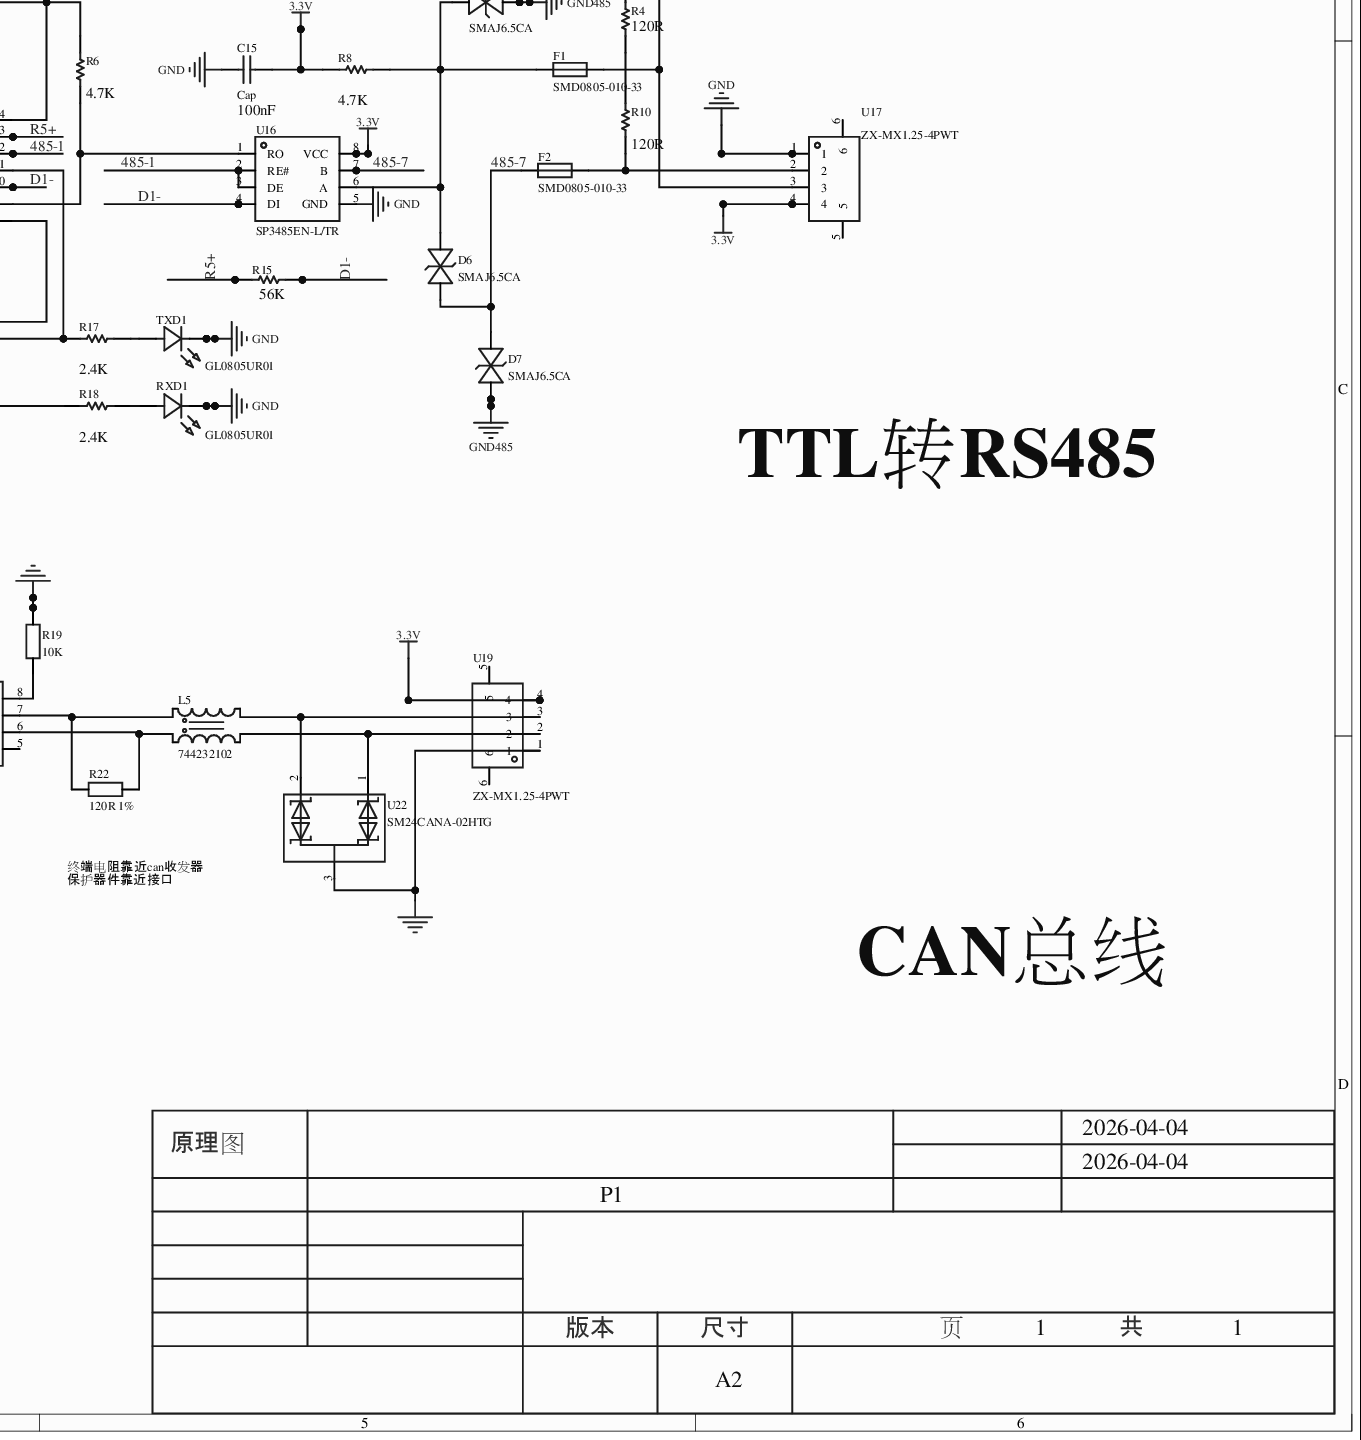
[diagram p0: MISC51972-3.schdoc, bottom right]
# Altium project MISC51972-2.PrjPcb (part 2 of 3)

## Sheet MISC51972-3.schdoc
size 594 x 419 mm; Version: V1.0; @Project Name: MISC51972; @Page Count: 1; @Update Date: 2026-04-04; @Create Date: 2026-04-04; @Schematic Name: MISC51972; @Page No: 1; @Board Name: MISC51972; @Create Time: 12:41:26; @Update Time: 16:32:51

### Parts
C1  100nF  [C0402]
C2  100nF  [C0402]
C3  100nF  [C0402]
C4  100nF  [C0402]
C5  100nF  [C0402]
C6  100nF  [C0402]
C7  100nF  [C0402]
C8  100nF  [C0402]
C9  12pF  [C0402]
C10  12pF  [C0402]
C11  100nF  [C0402]
C12  100nF  [C0402]
C13  100nF  [C0402]
C14  100nF  [C0402]
C15  Cap  value 100nF  [C0402]
C16  100nF  [C0402]
C17  100nF  [C0402]
C18  100nF  [C0402]
C19  100nF  [C0402]
C20  100nF  [C0402]
C21  Cap  value 1nF  [C0402]
C22  100nF  [C0402]
C23  22uF  [C0402]
C24  22uF  [C0402]
C25  100nF  [C0402]
C27  10uF  [C0402]
C28  22uF  [C0402]
C29  100nF  [C0603]
C30  47uF  [C1206]
C31  220uF  [CAP-SMD_BD6.3-L6.5-W6.5-LS7.2-FD]
C32  100uF  [CAP-SMD_BD6.3-L6.5-W6.5-LS7.0-FD]
C33  4.7uF  [C0603]
C34  100nF  [C0603]
C35  10uF  [C0402]
C36  22uF  [C0402]
C37  4.7nF  [C0603]
D1  CD143A-SR05  [SOT-143_L2.9-W1.3-P1.92-LS2.3-BL]
D2  CD143A-SR05  [SOT-143_L2.9-W1.3-P1.92-LS2.3-BL]
D3  CD143A-SR05  [SOT-143_L2.9-W1.3-P1.92-LS2.3-BL]
D4  CD143A-SR05  [SOT-143_L2.9-W1.3-P1.92-LS2.3-BL]
D5  SMAJ6.5CA  [SMA-L4.3-W2.6-LS5.3-BI]
D6  SMAJ6.5CA  [SMA-L4.3-W2.6-LS5.3-BI]
D7  SMAJ6.5CA  [SMA-L4.3-W2.6-LS5.3-BI]
D8  LL4148  [LL-34_L3.5-W1.5-RD]
D9  SS54  [SMA_L4.4-W2.8-LS5.4-R-RD]
D10  SS54  [SMA_L4.4-W2.8-LS5.4-R-RD]
DC1  DC-005-A200  [DC-IN-TH_DC-005-A200]
F1  SMD0805-010-33  [F0805]
F2  SMD0805-010-33  [F0805]
H1  PZ254V-11-04P  [HDR-TH_4P-P2.54-V-M]
H2  PZ254V-11-04P  [HDR-TH_4P-P2.54-V-M]
L1  DLM11SN900HY2L  [FILTER-SMD_4P-L1.3-W1.0-TL_DLP11SN201HL2L]
L2  DLM11SN900HY2L  [FILTER-SMD_4P-L1.3-W1.0-TL_DLP11SN201HL2L]
L3  DLM11SN900HY2L  [FILTER-SMD_4P-L1.3-W1.0-TL_DLP11SN201HL2L]
L4  DLM11SN900HY2L  [FILTER-SMD_4P-L1.3-W1.0-TL_DLP11SN201HL2L]
L5  744232102  [IND-SMD_4P-L3.2-W1.6]
L6  3.3uH  [IND-SMD_L7.0-W6.6]
L7  4.7uH  Rated Current: 5A  [IND-SMD_L7.0-W6.6]
LED1  15-21VGC/TR8  [LED0603_GREEN]  (value not drawn)
R1  0R  [R0402]
R2  0R  [R0402]
R3  9.53K  [R0402]
R4  value 120R  [R0402]  (hidden comment: Res1)
R5  value 4.7K  [R0402]  (hidden comment: Res1)
R6  value 4.7K  [R0402]  (hidden comment: Res1)
R7  90.9K  [R0402]
R8  value 4.7K  [R0402]  (hidden comment: Res1)
R9  10K  [R0402]
R10  value 120R  [R0402]  (hidden comment: Res1)
R11  4.7K  [R0402]
R12  4.7K  [R0402]
R13  4.7K  [R0402]
R14  4.7K  [R0402]
R15  value 56K  [R0402]  (hidden comment: Res1)
R16  value 4.7K  [R0402]  (hidden comment: Res1)
R17  value 2.4K  [R0402]  (hidden comment: Res1)
R18  value 2.4K  [R0402]  (hidden comment: Res1)
R19  10K  [R0402]
R20  10kΩ  [R0402]
R21  4.3kΩ  [R0402]
R22  120R 1%  [R0402]
R23  10kΩ  [R0402]
R24  51kΩ  [R0402]
R25  4.7kΩ  [R0402]
R26  1.5kΩ  [R0402]
R27  200kΩ  [R0402]
R28  10kΩ  [R0402]
R29  20kΩ  [R0402]
RXD1  GL0805UR01  [LED0805-R-RD_RED]
TXD1  GL0805UR01  [LED0805-R-RD_RED]
U1  TXS0102DCUT  [VSSOP-8_L2.3-W2.0-P0.50-LS3.1-BR]
U2  TPS2060CDGNR  [HVSSOP-8_L3.0-W3.0-P0.65-LS4.9-BL-EP-1]
U3  (no value)  [PCMF2USB3S]
U4  (no value)  [tp点]
U5  (no value)  [PCMF2USB3S]
U6  (no value)  [tp点]
U7  TXS0102DCUT  [VSSOP-8_L2.3-W2.0-P0.50-LS3.1-BR]
U8  TPS2060CDGNR  [HVSSOP-8_L3.0-W3.0-P0.65-LS4.9-BL-EP-1]
U9  (no value)  [PCMF2USB3S]
U10  (no value)  [tp点]
U11  (no value)  [PCMF2USB3S]
U12  (no value)  [tp点]
U13  HC-USB3.0-L168-WP  [USB-TH_USB3.0-A]
U14  TUSB8041IRGCR  [QFN-64_L9.0-W9.0-P0.50-BL-EP7.2]
U15  74HC04D,653  [SOIC-14_L8.7-W3.9-P1.27-LS6.0-BL]
U16  SP3485EN-L/TR  [SOIC-8_L5.0-W4.0-P1.27-LS6.0-BL]
U17  ZX-MX1.25-4PWT  [CONN-SMD_4P-P1.25-MX1.25-4P-WT]
U18  SN65HVD230DR  [SOIC-8_L4.9-W3.9-P1.27-LS6.0-BL]
U19  ZX-MX1.25-4PWT  [CONN-SMD_4P-P1.25-MX1.25-4P-WT]
U20  AMS1117-1.8  [SOT-223-4_L6.5-W3.5-P2.30-LS7.0-BR]
U21  TPS563201DDCR  [SOT-23-6_L2.9-W1.6-P0.95-LS2.8-BR]
U22  SM24CANA-02HTG  [SOT-23-3_L2.9-W1.3-P1.90-LS2.4-BR]
U23  SCT2450STER  [ESOP-8_L4.9-W3.9-P1.27-LS6.0-BL-EP]
U24  AMS1117-3.3  [SOT-223-4_L6.5-W3.5-P2.30-LS7.0-BR]
USB1  HC-USB3.0-L175-2X1-P  [USB-A-TH_H181-AF2R06-12ALCR]
USB2  HC-USB3.0-L175-2X1-P  [USB-A-TH_H181-AF2R06-12ALCR]
X1  24MHz  [CRYSTAL-SMD_4P-L3.2-W2.5-BL]

### Ports
USB30_SSRXM (in), USB30_SSRXP (in), USB30_SSTXM (in), USB30_SSTXP (in), USB30_USB_DM (in), USB30_USB_DP (in)

### Nets
1.1V: C11.2 C12.2 C13.2 C14.2 C16.2 C18.2 C19.2 C20.2 C23.2 C24.2 C25.2 L6.1 R21.2 U14.5(VDD) U14.8(VDD) U14.13(VDD) U14.21(VDD) U14.28(VDD) U14.31(VDD) U14.51(VDD) U14.57(VDD)
1.8V: C3.1 C6.1 C28.2 U1.3(VCCA) U1.4(A2) U1.5(A1) U7.3(VCCA) U7.4(A2) U7.5(A1) U20.2(Out) U20.4(TAB)
3.3V: C15.1 C36.2 H1.4 H2.1 R5.2 R6.2 R8.2 R14.2 U14.16(VDD33) U14.34(VDD33) U14.52(VDD33) U14.63(VDD33) U15.14(VCC) U16.8(VCC) U17.4 U18.3(VCC) U19.4 U24.2(VOUT(TAB)) U24.4(TAB)
12V: C27.2 D10.1(A) DC1.1 U20.3(In)
D5.0V: C1.2 C2.1 C4.2 C5.1 C35.2 D9.2(K) R7.2 R20.2 R24.1 R25.1 U1.6(OE) U1.7(VCCB) U2.2(IN) U7.6(OE) U7.7(VCCB) U8.2(IN) U13.1(VBUS) U21.3(VIN) U24.3(VIN)
GND: C1.1 C2.2 C3.2 C4.1 C5.2 C6.2 C9.1 C10.1 C11.1 C12.1 C13.1 C14.1 C15.2 C16.1 C17.2 C18.1 C19.1 C20.1 C21.1 C23.1 C24.1 C25.1 C27.1 C28.1 C30.1 C31.2 C32.2 C33.1 C34.1 C35.1 C36.1 C37.2 D1.1(GND) D2.1(GND) D3.1(GND) D4.1(GND) DC1.2 H1.1 H2.4 LED1.2(C) R3.2 R9.2 R11.2 R12.2 R13.2 R16.1 R19.2 R23.2 R27.1 R28.2 RXD1.2(C) TXD1.2(C) U1.2(GND) U2.1(GND) U2.9(EP) U3.B1(6) U3.B2(5) U5.B1(6) U5.B2(5) U7.2(GND) U8.1(GND) U8.9(EP) U9.B1(6) U9.B2(5) U11.B1(6) U11.B2(5) U13.4(GND) U13.7(GND_DRAN) U13.10(SH) U14.65(VSS) U15.7(GND) U16.5(GND) U17.1 U18.2(GND) U19.1 U20.1(GND) U21.1(GND) U22.3 U23.7(GND) U23.9(EP) U24.1(ADJ(GND)) USB1.4(GND) USB1.7(GND_DRAIN) USB1.13(GND) USB1.16(GND_DRAIN) USB1.19(GND) USB1.20(GND) USB2.4(GND) USB2.7(GND_DRAIN) USB2.13(GND) USB2.16(GND_DRAIN) USB2.19(GND) USB2.20(GND) X1.2(GND) X1.4(GND)
GND485: D5.2 D7.1
USB5_5V: D2.4(REF) U2.7(OUT1) USB1.10(VBUS)
USB6_5V: D1.4(REF) U2.6(OUT2) USB1.1(VBUS)
USB7_5V: D4.4(REF) U8.7(OUT1) USB2.10(VBUS)
USB8_5V: D3.4(REF) U8.6(OUT2) USB2.1(VBUS)
485-1: U15.12(6Y) U16.2(RE#) U16.3(DE)
485-7: D6.1 D7.2 F2.1 R16.2 U16.7(B)
D1-: D8.1(C) R15.1 U15.10(5Y) U16.4(DI)
P74_TXD6: H1.3 R5.1 U15.1(1A)
P75_RXD6: H1.2 U15.4(2Y) U15.5(3A)
P84_CAN_TX2: H2.3 U18.1(D)
P85_CAN_RX2: H2.2 U18.4(R)
R5+: C21.2 D8.2(A) R15.2 U15.13(6A)
USB30_SSRXM: U14.56(USB_SSTXM_UP)
USB30_SSRXP: U14.55(USB_SSTXP_UP)
USB30_SSTXM: C8.2 U14.59(USB_SSRXM_UP) ; port USB30_SSTXM
USB30_SSTXP: C7.2 U14.58(USB_SSRXP_UP) ; port USB30_SSTXP
USB30_T_DM1: L1.1 U14.2(USB_DM_DN1)
USB30_T_DM2: L2.1 U14.10(USB_DM_DN2)
USB30_T_DM3: L3.1 U14.18(USB_DM_DN3)
USB30_T_DM4: L4.1 U14.25(USB_DM_DN4)
USB30_T_DP1: L1.4 U14.1(USB_DP_DN1)
USB30_T_DP2: L2.4 U14.9(USB_DP_DN2)
USB30_T_DP3: L3.4 U14.17(USB_DP_DN3)
USB30_T_DP4: L4.4 U14.24(USB_DP_DN4)
USB30_T_SSRXM1: U5.A4(11) U14.7(USB_SSRXM_DN1)
USB30_T_SSRXM2: U3.A4(11) U14.15(USB_SSRXM_DN2)
USB30_T_SSRXM3: U11.A4(11) U14.23(USB_SSRXM_DN3)
USB30_T_SSRXM4: U9.A4(11) U14.30(USB_SSRXM_DN4)
USB30_T_SSRXP1: U5.A3(10) U14.6(USB_SSRXP_DN1)
USB30_T_SSRXP2: U3.A3(10) U14.14(USB_SSRXP_DN2)
USB30_T_SSRXP3: U11.A3(10) U14.22(USB_SSRXP_DN3)
USB30_T_SSRXP4: U9.A3(10) U14.29(USB_SSRXP_DN4)
USB30_T_SSTXM1: U5.A2(8) U14.4(USB_SSTXM_DN1)
USB30_T_SSTXM2: U3.A2(8) U14.12(USB_SSTXM_DN2)
USB30_T_SSTXM3: U11.A2(8) U14.20(USB_SSTXM_DN3)
USB30_T_SSTXM4: U9.A2(8) U14.27(USB_SSTXM_DN4)
USB30_T_SSTXP1: U5.A1(7) U14.3(USB_SSTXP_DN1)
USB30_T_SSTXP2: U3.A1(7) U14.11(USB_SSTXP_DN2)
USB30_T_SSTXP3: U11.A1(7) U14.19(USB_SSTXP_DN3)
USB30_T_SSTXP4: U9.A1(7) U14.26(USB_SSTXP_DN4)
USB30_USB_DM: U14.54(USB_DM_UP)
USB30_USB_DP: U14.53(USB_DP_UP)
NetC7_1: C7.1 U13.9(SSTX+)
NetC8_1: C8.1 U13.8(SSTX-)
NetC9_2: C9.2 U14.62(XI) X1.1(OSC1)
NetC10_2: C10.2 U14.61(XO) X1.3(OSC2)
NetC17_1: C17.1 U14.50(GRSTz)
NetC22_1: C22.1 L6.2 U21.2(SW)
NetC22_2: C22.2 U21.6(VBST)
NetC29_1: C29.1 L7.1 U23.8(SW)
NetC29_2: C29.2 U23.1(BOOT)
NetC30_2: C30.2 C31.1 D9.1(A) L7.2
NetC32_1: C32.1 C33.2 C34.2 D10.2(K) U23.2(VIN) U23.3(EN)
NetC37_1: C37.1 R29.2
NetD1_2: D1.2(I/O) L1.2 USB1.2(D-)
NetD1_3: D1.3(I/O) L1.3 USB1.3(D+)
NetD2_2: D2.2(I/O) L2.2 USB1.11(D-)
NetD2_3: D2.3(I/O) L2.3 USB1.12(D+)
NetD3_2: D3.2(I/O) L3.2 USB2.2(D-)
NetD3_3: D3.3(I/O) L3.3 USB2.3(D+)
NetD4_2: D4.2(I/O) L4.2 USB2.11(D-)
NetD4_3: D4.3(I/O) L4.3 USB2.12(D+)
NetD5_1: D5.1 D6.2 F1.1 R8.1 U16.6(A)
NetF1_2: F1.2 R4.1 U17.3
NetF2_2: F2.2 R10.1 U17.2
NetL5_1: L5.1 R22.1 U18.6(CANL)
NetL5_2: L5.2 U19.2 U22.1
NetL5_3: L5.3 U19.3 U22.2
NetL5_4: L5.4 R22.2 U18.7(CANH)
NetLED1_1: LED1.1(A) R25.2
NetR1_1: R1.1 U13.6(SSRX+)
NetR1_2: R1.2 ; port USB30_SSRXP
NetR2_1: R2.1 U13.5(SSRX-)
NetR2_2: R2.2 ; port USB30_SSRXM
NetR3_1: R3.1 U14.64(USB_R1)
NetR4_2: R4.2 R10.2
NetR6_1: R6.1 U15.9(4A) U16.1(RO)
NetR7_1: R7.1 R9.1 U14.48(USB_VBUS)
NetR11_1: R11.1 U14.49(TEST)
NetR12_1: R12.1 U14.45(AUTOENz/HS_SUSPEND)
NetR13_1: R13.1 U14.42(GANGED/SMBA2/HS_UP)
NetR14_1: R14.1 U14.40(FULLPWRMGMTz/SMBA1/SS_UP)
NetR17_1: R17.1 U15.2(1Y) U15.11(5A)
NetR17_2: R17.2 TXD1.1(A)
NetR18_1: R18.1 RXD1.1(A)
NetR18_2: R18.2 U15.6(3Y)
NetR19_1: R19.1 U18.8(RS)
NetR20_1: R20.1 U21.5(EN)
NetR21_1: R21.1 R23.1 U21.4(VFB)
NetR24_2: R24.2 R26.1
NetR26_2: R26.2 R28.1 U23.5(FB)
NetR27_2: R27.2 U23.4(RT/CLK)
NetR29_1: R29.1 U23.6(COMP)
NetU1_1: U1.1(B2) U2.3(EN1orEN1#)
NetU1_8: U1.8(B1) U2.4(EN2orEN2#)
NetU2_5: U2.5(FLT2#) U6.1
NetU2_8: U2.8(FLT1#) U4.1
NetU3_C1: U3.C1(1) USB1.18(SSTX+)
NetU3_C2: U3.C2(2) USB1.17(SSTX-)
NetU3_C3: U3.C3(3) USB1.15(SSRX+)
NetU3_C4: U3.C4(4) USB1.14(SSRX-)
NetU5_C1: U5.C1(1) USB1.9(SSTX+)
NetU5_C2: U5.C2(2) USB1.8(SSTX-)
NetU5_C3: U5.C3(3) USB1.6(SSRX+)
NetU5_C4: U5.C4(4) USB1.5(SSRX-)
NetU7_1: U7.1(B2) U8.3(EN1orEN1#)
NetU7_8: U7.8(B1) U8.4(EN2orEN2#)
NetU8_5: U8.5(FLT2#) U12.1
NetU8_8: U8.8(FLT1#) U10.1
NetU9_C1: U9.C1(1) USB2.18(SSTX+)
NetU9_C2: U9.C2(2) USB2.17(SSTX-)
NetU9_C3: U9.C3(3) USB2.15(SSRX+)
NetU9_C4: U9.C4(4) USB2.14(SSRX-)
NetU11_C1: U11.C1(1) USB2.9(SSTX+)
NetU11_C2: U11.C2(2) USB2.8(SSTX-)
NetU11_C3: U11.C3(3) USB2.6(SSRX+)
NetU11_C4: U11.C4(4) USB2.5(SSRX-)
NetU13_2: U13.2(D-) ; port USB30_USB_DM
NetU13_3: U13.3(D+) ; port USB30_USB_DP
NetU15_3: U15.3(2A) U15.8(4Y)

Not connected (* = marked no-connect by the designer): DC1 3; U14 32(PWRCTL4/BATEN4)* 33(PWRCTL3/BATEN3)* 35(PWRCTL2/BATEN2)* 36(PWRCTL1/BATEN1)* 37(SDA/SMBDAT)* 38(SCL/SMBCLK)* 39(SMBUSz/SS_SUSPEND)* 41(PWRCTL_POL)* 43(OVERCUR4z)* 44(OVERCUR3z)* 46(OVERCUR1z)* 47(OVERCUR2z)* 60(NC)*; U17 5 6; U18 5(VREF)*; U19 5 6

### Notes on the sheet
- 热插拔控制器
- 双路USB3.0
- USB3.0拓展
- TTL转RS485
- (near R23) 1.1V电源模块
- 终端电阻靠近can收发器
  保护器件靠近接口
- 1.8V电源模块
- CAN总线
- 5V电源模块
- 3.3V电源模块
- 2026-04-04
- 原理图
- P1
- 版本
- 尺寸
- A2
- 页
- 1
- 共